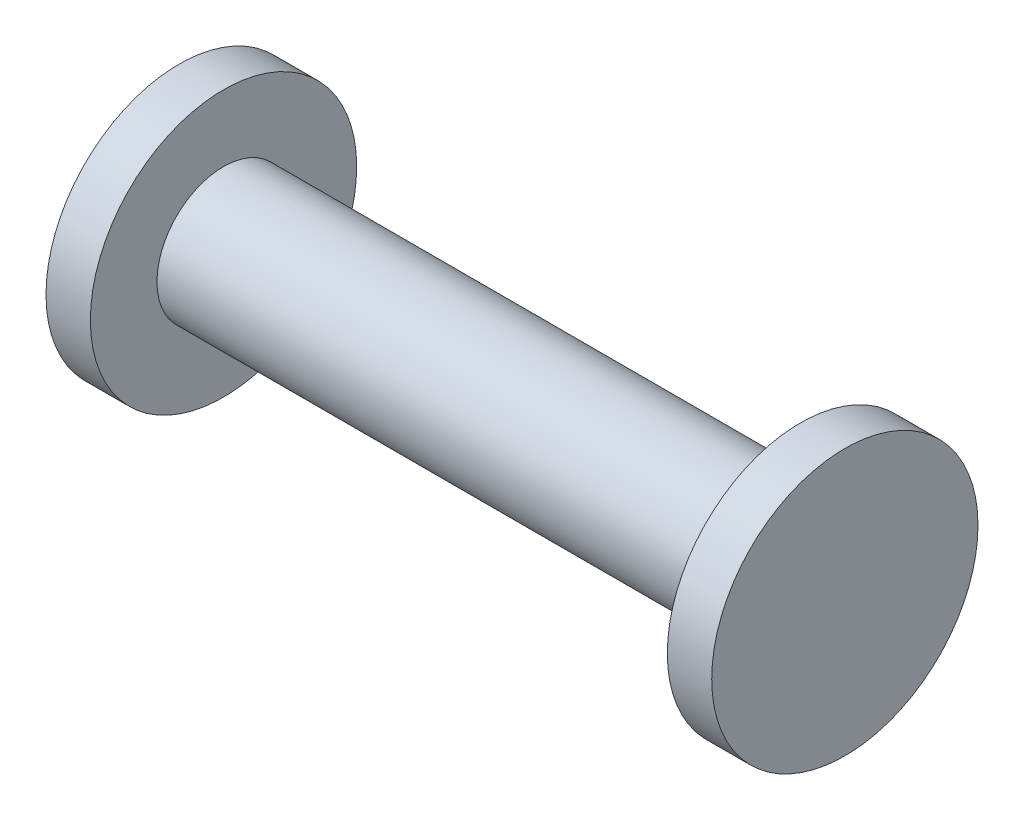
SolidWorks part; units mm, degrees
ref_plane "Front Plane" through (0, 0, 0) normal (0, 0, 1) x (1, 0, 0)
ref_plane "Top Plane" through (0, 0, 0) normal (0, 1, 0) x (1, 0, 0)
ref_plane "Right Plane" through (0, 0, 0) normal (1, 0, 0) x (0, 0, -1)
sketch "Sketch3" plane through (0, 0, 0) normal (0, 0, 1) x (1, 0, 0)
  line L0 (-37.5, 0) -> (37.5, 0)
  line L1 (37.5, 0) -> (37.5, 15)
  line L2 (37.5, 15) -> (32.5, 15)
  line L3 (32.5, 15) -> (32.5, 7.5)
  line L4 (32.5, 7.5) -> (-32.5, 7.5)
  line L5 (-32.5, 7.5) -> (-32.5, 15)
  line L6 (-32.5, 15) -> (-37.5, 15)
  line L7 (-37.5, 15) -> (-37.5, 0)
revolve "Revolve1" add sketch "Sketch3" angle 360 about L0
scale "Scale1" scale about origin uniform scaling yes scale factor 0.3
